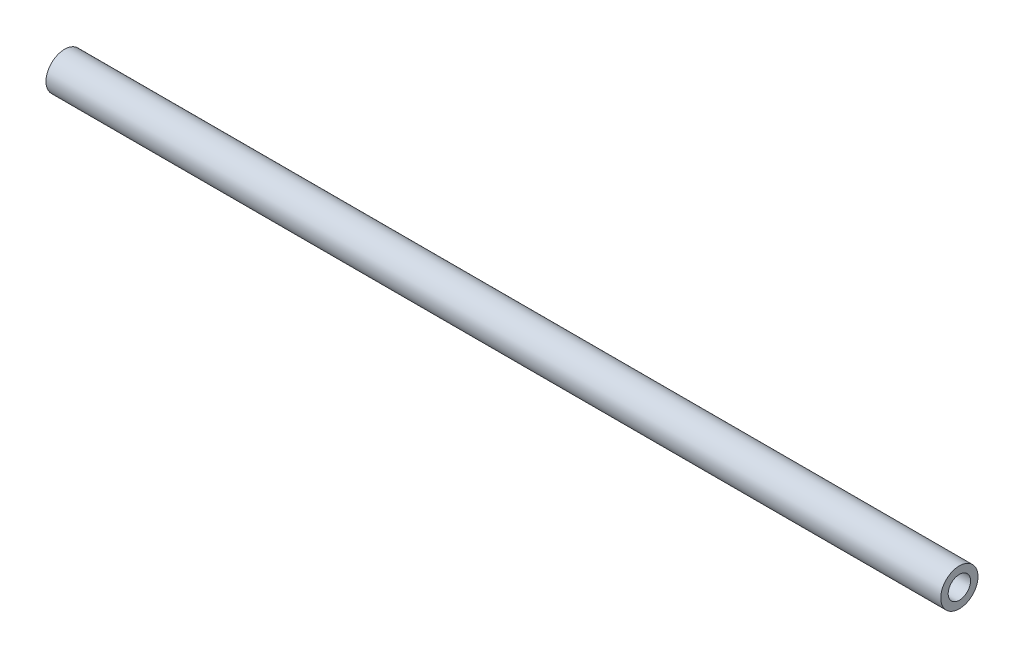
SolidWorks part; units mm, degrees
ref_plane "前视基准面" through (0, 0, 0) normal (0, 0, 1) x (1, 0, 0)
ref_plane "上视基准面" through (0, 0, 0) normal (0, 1, 0) x (1, 0, 0)
ref_plane "右视基准面" through (0, 0, 0) normal (1, 0, 0) x (0, 0, -1)
sketch "草图1" plane through (0, 0, 0) normal (1, 0, 0) x (0, 0, -1)
  circle A0 centre (0, 0) radius 2.5
  circle A1 centre (0, 0) radius 1.5
  dimension "D1" = 3
  dimension "D2" = 5
extrude "凸台-拉伸1" add sketch "草图1" along normal blind 120
